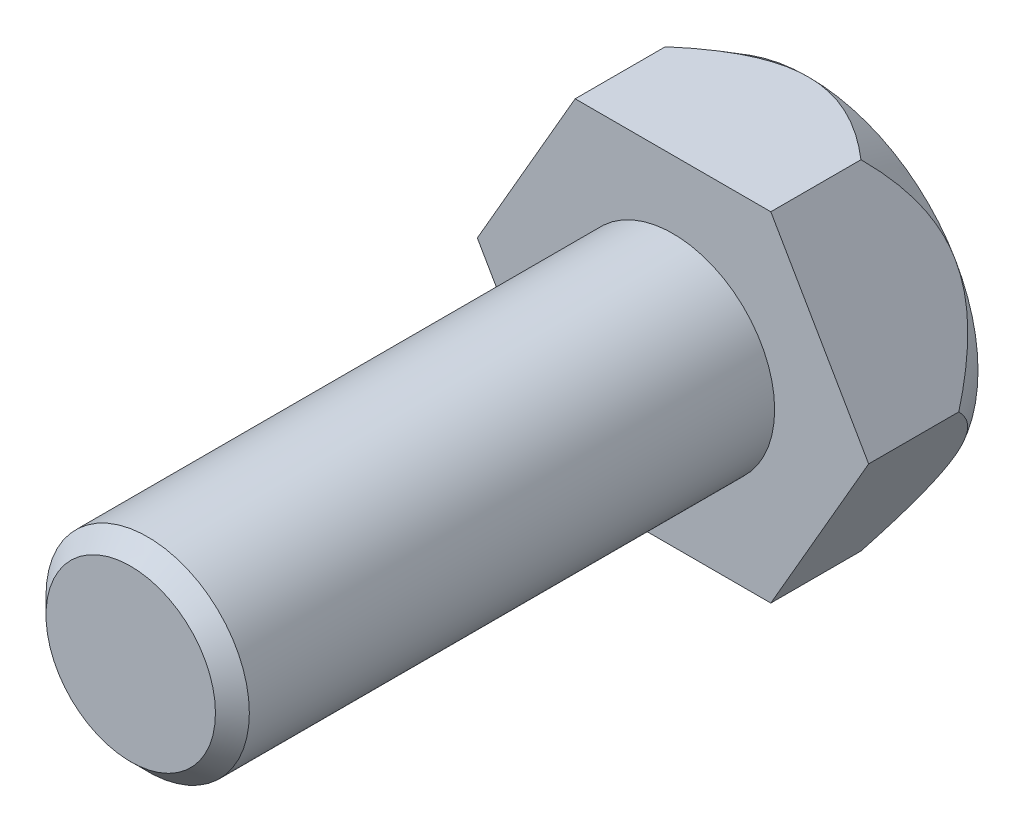
from build123d import *

# Parameters (mm, degrees)
BOSS_EXTRUDE1_DEPTH = 4
SKETCH2_OUTSIDE_W   = 21.324
SKETCH2_OUTSIDE_H   = 19.776
SKETCH2_OUTSIDE_R   = 5
CUT_EXTRUDE1_DEPTH  = 4
CUT_EXTRUDE1_DRAFT  = -30
SKETCH3_R           = 3
BOSS_EXTRUDE2_DEPTH = 16
CHAMFER1_SIZE       = 0.5


with BuildPart() as part:
    # Sketch1 → Boss-Extrude1 (new body)
    with BuildSketch(Plane.XY):
        Polygon((2.886751346, 5), (-2.886751346, 5), (-5.773502692, 0), (-2.886751346, -5), (2.886751346, -5), (5.773502692, 0), align=None)
    extrude(amount=BOSS_EXTRUDE1_DEPTH)


with BuildPart() as cut_extrude1_tool:
    # Sketch2 outside → Cut-Extrude1 (with draft: the straight prism first)
    with BuildSketch(Plane(origin=(0, 0, 0), x_dir=(-1, 0, 0), z_dir=(0, 0, -1))):
        Rectangle(SKETCH2_OUTSIDE_W, SKETCH2_OUTSIDE_H)
        Circle(SKETCH2_OUTSIDE_R, mode=Mode.SUBTRACT)
    extrude(amount=-CUT_EXTRUDE1_DEPTH)
    # Cut-Extrude1: the draft: its side faces are tilted about the plane it starts from
    cut_extrude1_sides = [cut_extrude1_tool.faces().sort_by_distance(p)[0] for p in [
        (0, -9.888, 2),
        (-10.662, 0, 2),
        (0, 9.888, 2),
        (10.662, 0, 2),
        (5, 0, 2),
    ]]
    draft(cut_extrude1_sides, Plane(origin=(0, 0, 0), x_dir=(-1, 0, 0), z_dir=(0, 0, -1)), CUT_EXTRUDE1_DRAFT)


with BuildPart() as part_1:
    add(part.part)

    # Cut-Extrude1: cut by cut_extrude1_tool
    add(cut_extrude1_tool.part, mode=Mode.SUBTRACT)

    # Sketch3 → Boss-Extrude2 (add)
    with BuildSketch(Plane.XY.offset(4)):
        Circle(SKETCH3_R)
    extrude(amount=BOSS_EXTRUDE2_DEPTH)

    # Chamfer1
    chamfer1_edges = [part_1.edges().sort_by_distance(p)[0] for p in [
        (-3, 0, 20),
    ]]
    chamfer(chamfer1_edges, length=CHAMFER1_SIZE)


solid = part_1.part
